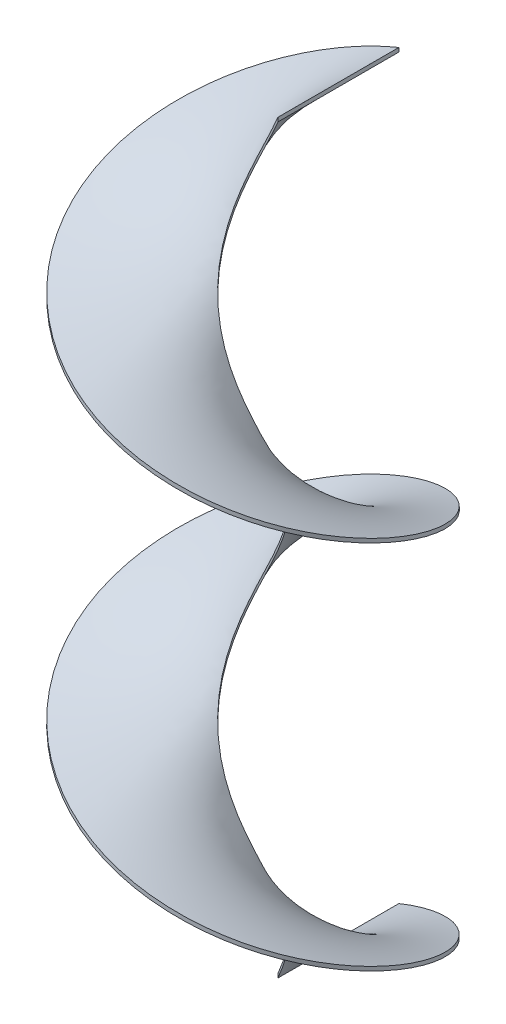
from build123d import *

# Parameters (mm, degrees)
SWEEP_14_PITCH       = 230
SWEEP_14_HEIGHT      = 460
SWEEP_14_RADIUS      = 15
SWEEP_14_START_ANGLE = -180
SKETCH_11_W          = 75
SKETCH_11_H          = 2.5


with BuildPart() as part:
    # 扫描14: sweep along a helix
    with BuildLine() as sweep_14_path:
        add(Helix(SWEEP_14_PITCH, SWEEP_14_HEIGHT, SWEEP_14_RADIUS, center=(0, 0, 0), direction=(0, 1, 0), lefthand=True, mode=Mode.PRIVATE).rotate(Axis((0, 0, 0), (0, 1, 0)), SWEEP_14_START_ANGLE))
    # 草图11 → 扫描14 (sweep)
    with BuildSketch(Plane(origin=(0, 0, 0), x_dir=(0, 0, -1), z_dir=(1, 0, 0))):
        with Locations((53, 0)):
            Rectangle(SKETCH_11_W, SKETCH_11_H)
    sweep(path=sweep_14_path.line, is_frenet=True)


solid = part.part
